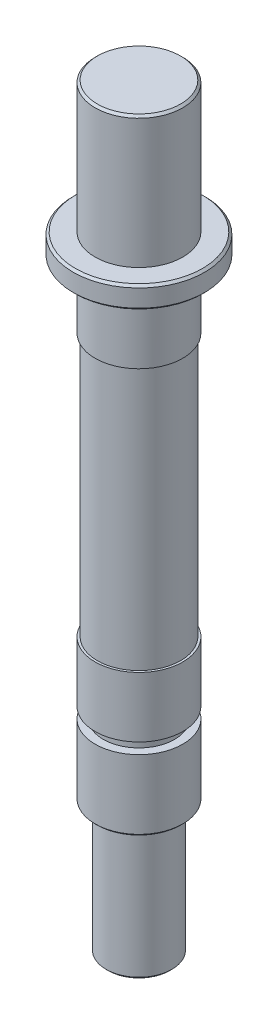
from build123d import *

# Parameters (mm, degrees)
SKETCH1_R           = 4
BOSS_EXTRUDE1_DEPTH = 43
SKETCH2_R           = 6
BOSS_EXTRUDE2_DEPTH = 2
SKETCH10_R          = 4
BOSS_EXTRUDE4_DEPTH = 12
SKETCH8_W           = 4.085685727
SKETCH8_H           = 24
SKETCH8_W_2         = 3.929787065
SKETCH8_H_2         = 1
SKETCH9_R           = 3
BOSS_EXTRUDE3_DEPTH = 12
CHAMFER1_SIZE       = 0.2


with BuildPart() as part:
    # Sketch1 → Boss-Extrude1 (new body)
    with BuildSketch(Plane(origin=(0, 0, 0), x_dir=(1, 0, 0), z_dir=(0, 1, 0))):
        with Locations(Location((0, 0, 0), (0, 0, 270))):
            Circle(SKETCH1_R)
    extrude(amount=BOSS_EXTRUDE1_DEPTH)

    # Sketch2 → Boss-Extrude2 (add)
    with BuildSketch(Plane(origin=(0, 43, 0), x_dir=(1, 0, 0), z_dir=(0, 1, 0))):
        with Locations(Location((0, 0, 0), (0, 0, 270))):
            Circle(SKETCH2_R)
    extrude(amount=BOSS_EXTRUDE2_DEPTH)

    # Sketch10 → Boss-Extrude4 (add)
    with BuildSketch(Plane(origin=(0, 45, 0), x_dir=(1, 0, 0), z_dir=(0, 1, 0))):
        with Locations(Location((0, 0, 0), (0, 0, 270))):
            Circle(SKETCH10_R)
    extrude(amount=BOSS_EXTRUDE4_DEPTH)

    # Sketch8 → Cut-Revolve1 (revolve, cut)
    with BuildSketch(Plane.XY):
        with Locations((5.842842864, 25)):
            Rectangle(SKETCH8_W, SKETCH8_H)
        with Locations((5.214893532, 7)):
            Rectangle(SKETCH8_W_2, SKETCH8_H_2)
    revolve(axis=Axis((0, 0, 0), (0, 1, 0)), mode=Mode.SUBTRACT)

    # Sketch9 → Boss-Extrude3 (add)
    with BuildSketch(Plane.XZ):
        with Locations(Location((0, 0, 0), (0, 0, 90))):
            Circle(SKETCH9_R)
    extrude(amount=BOSS_EXTRUDE3_DEPTH)

    # Chamfer1
    chamfer1_edges = [part.edges().sort_by_distance(p)[0] for p in [
        (0, 57, -4),
        (0, 0, -4),
        (0, -12, -3),
        (0, 43, -6),
        (0, 45, -6),
    ]]
    chamfer(chamfer1_edges, length=CHAMFER1_SIZE)


solid = part.part
